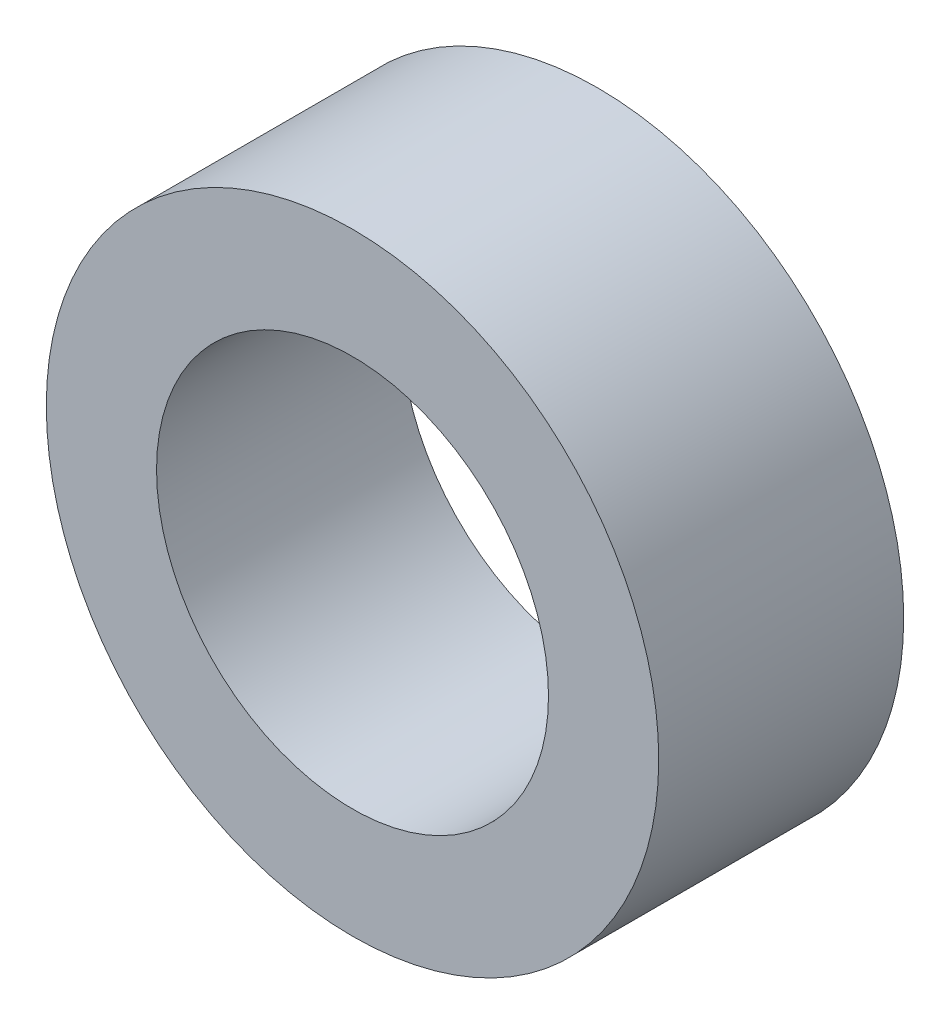
SolidWorks part; units mm, degrees
ref_plane "前视基准面" through (0, 0, 0) normal (0, 0, 1) x (1, 0, 0)
ref_plane "上视基准面" through (0, 0, 0) normal (0, 1, 0) x (1, 0, 0)
ref_plane "右视基准面" through (0, 0, 0) normal (1, 0, 0) x (0, 0, -1)
sketch "草图1" plane through (0, 0, 0) normal (0, 0, 1) x (1, 0, 0)
  circle A0 centre (0, 0) radius 8
  circle A1 centre (0, 0) radius 12.5
  dimension "D1" = 16
  dimension "D2" = 25
extrude "凸台-拉伸1" add sketch "草图1" along normal mid plane 10
